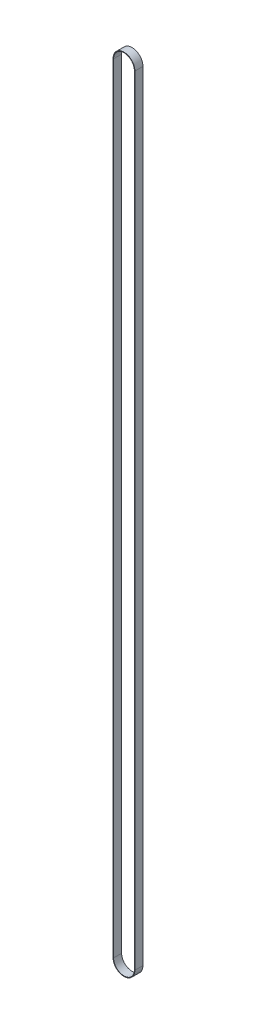
from build123d import *

# Parameters (mm, degrees)
EXTRUDE_1_DEPTH = 7.5


with BuildPart() as part:
    # 草图2 → 拉伸-薄壁1 (new, symmetric)
    with BuildSketch(Plane.XY):
        with BuildLine():
            Line((20.415, 1455), (20.415, 0))
            ThreePointArc((20.415, 0), (0, -20.415), (-20.415, 0))
            Line((-20.415, 0), (-20.415, 1455))
            ThreePointArc((-20.415, 1455), (0, 1475.415), (20.415, 1455))
        make_face()
        with BuildLine():
            Line((19.415, 1455), (19.415, 0))
            ThreePointArc((19.415, 0), (0, -19.415), (-19.415, 0))
            Line((-19.415, 0), (-19.415, 1455))
            ThreePointArc((-19.415, 1455), (0, 1474.415), (19.415, 1455))
        make_face(mode=Mode.SUBTRACT)
    extrude(amount=EXTRUDE_1_DEPTH, both=True)


solid = part.part
